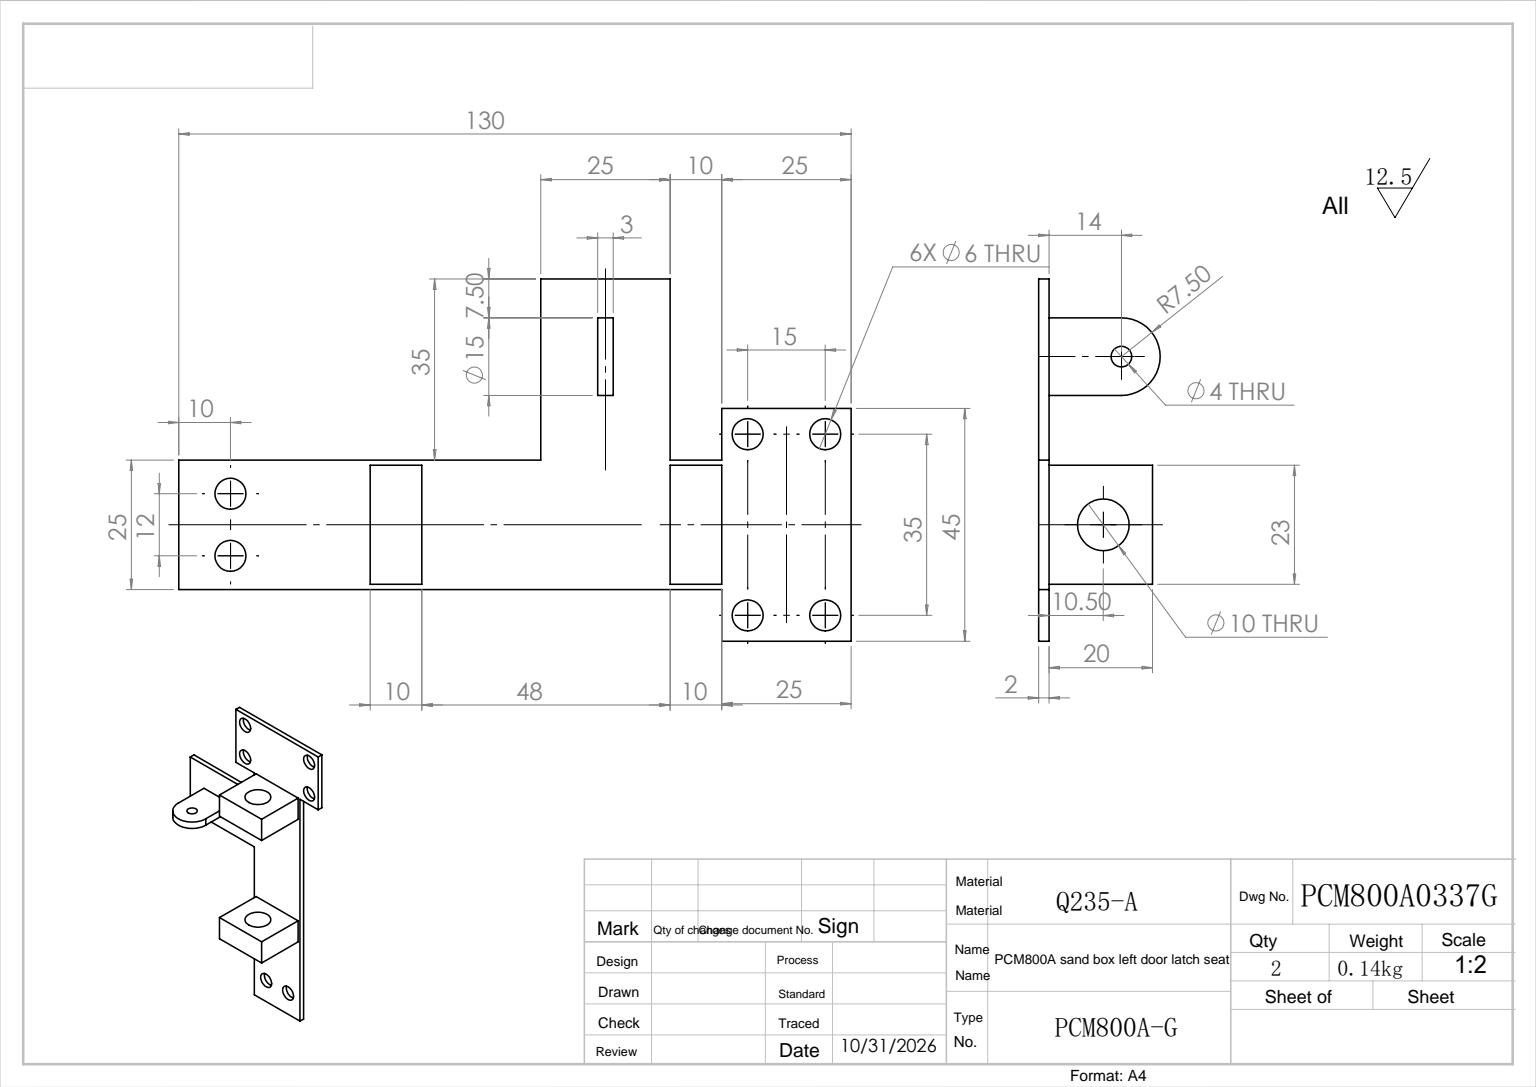
from build123d import *

# Parameters (mm, degrees)
SKETCH_1_R             = 3
EXTRUDE_1_DEPTH        = 2
EXTRUDE_START          = -25
SKETCH_2_W             = 23
SKETCH_2_H             = 20
SKETCH_2_R             = 5
EXTRUDE_2_DEPTH        = 10
PATTERN_LINEAR_1_COUNT = 2
PATTERN_LINEAR_1_PITCH = 58
EXTRUDE_START_2        = -11
SKETCH_3_R             = 2
EXTRUDE_3_DEPTH        = 3


with BuildPart() as part:
    # 草图1 → 凸台-拉伸1 (new body)
    with BuildSketch(Plane.XY):
        Polygon((0, 0), (45, 0), (45, -25), (35, -25), (35, -130), (10, -130), (10, -60), (-25, -60), (-25, -35), (10, -35), (10, -25), (0, -25), align=None)
        with Locations((5, -5)):
            Circle(SKETCH_1_R, mode=Mode.SUBTRACT)
        with Locations((40, -5)):
            Circle(SKETCH_1_R, mode=Mode.SUBTRACT)
        with Locations((5, -20)):
            Circle(SKETCH_1_R, mode=Mode.SUBTRACT)
        with Locations((40, -20)):
            Circle(SKETCH_1_R, mode=Mode.SUBTRACT)
        with Locations((16.5, -120)):
            Circle(SKETCH_1_R, mode=Mode.SUBTRACT)
        with Locations((28.5, -120)):
            Circle(SKETCH_1_R, mode=Mode.SUBTRACT)
    extrude(amount=EXTRUDE_1_DEPTH)

    # 草图2 → 凸台-拉伸2 (add)
    with BuildSketch(Plane(origin=(0, 0, 0), x_dir=(1, 0, 0), z_dir=(0, 1, 0)).offset(EXTRUDE_START)):
        with Locations((22.5, -12)):
            Rectangle(SKETCH_2_W, SKETCH_2_H)
        with Locations(Location((22.5, -12.5, 0), (0, 0, 270))):
            Circle(SKETCH_2_R, mode=Mode.SUBTRACT)
    extrude_2 = extrude(amount=-EXTRUDE_2_DEPTH)

    # 阵列(线性)1: 凸台-拉伸2 ×2
    with Locations(*[(0, -i * PATTERN_LINEAR_1_PITCH, 0) for i in range(1, PATTERN_LINEAR_1_COUNT)]):
        add(extrude_2)

    # 草图3 → 凸台-拉伸3 (add)
    with BuildSketch(Plane(origin=(0, -35, 0), x_dir=(1, 0, 0), z_dir=(0, 1, 0)).offset(EXTRUDE_START_2)):
        with BuildLine():
            Line((-17.5, -2), (-2.5, -2))
            Line((-2.5, -2), (-2.5, -16))
            ThreePointArc((-2.5, -16), (-10, -23.5), (-17.5, -16))
            Line((-17.5, -16), (-17.5, -2))
        make_face()
        with Locations(Location((-10, -16, 0), (0, 0, 270))):
            Circle(SKETCH_3_R, mode=Mode.SUBTRACT)
    extrude(amount=-EXTRUDE_3_DEPTH)


solid = part.part
